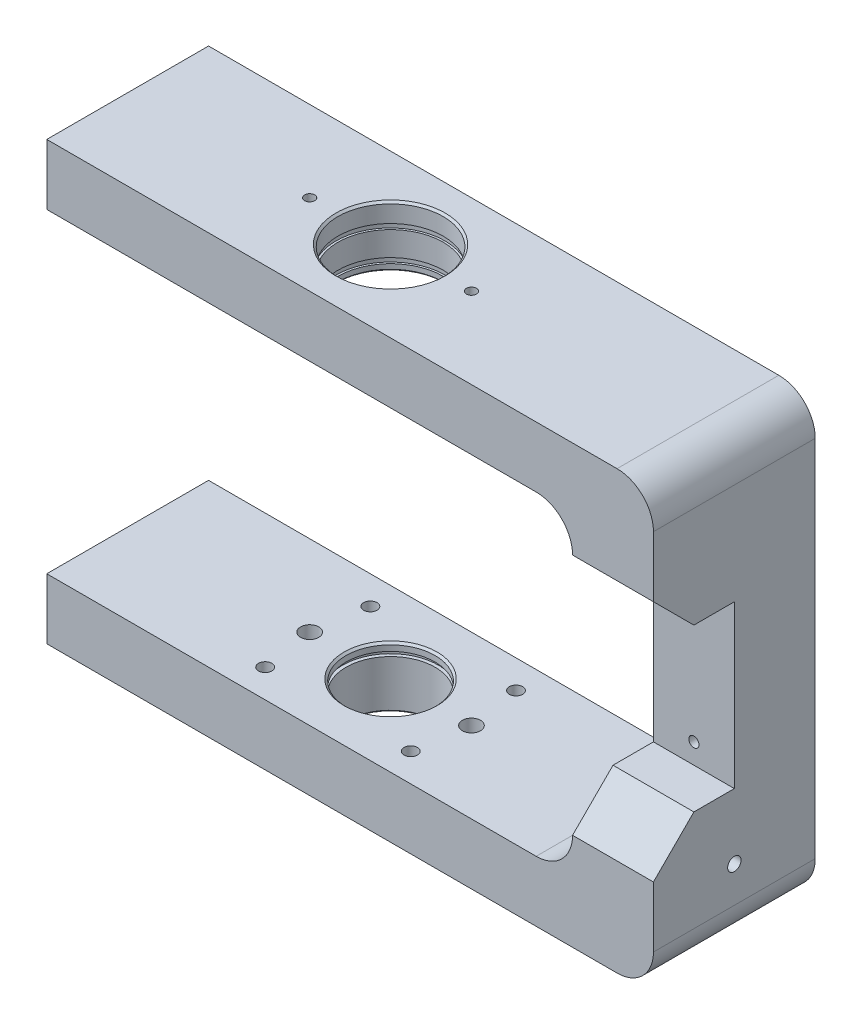
from build123d import *

# Parameters (mm, degrees)
BOSS_EXTRUDE1_DEPTH   = 40
SKETCH2_R             = 11
CUT_EXTRUDE1_DEPTH    = 190.1137224
SKETCH3_R             = 13
CUT_EXTRUDE2_DEPTH    = 40
SKETCH4_R             = 11.85
CUT_EXTRUDE3_DEPTH    = 1.1
SKETCH5_R             = 13.5
CUT_EXTRUDE4_DEPTH    = 1.3
LPATTERN1_COUNT       = 2
LPATTERN1_PITCH       = 7.3
M3_TAPPED_HOLE1_D     = 2.5
M3_TAPPED_HOLE1_DEPTH = 7.5
M3_TAPPED_HOLE1_TIP   = 0.751075774
CUT_EXTRUDE5_REACH    = 191.114
CHAMFER1_SIZE         = 0.5
M3_TAPPED_HOLE2_D     = 2.5
M3_TAPPED_HOLE2_DEPTH = 7.5
M3_TAPPED_HOLE2_TIP   = 0.751075774
M4_TAPPED_HOLE1_D     = 3.3
M4_TAPPED_HOLE1_DEPTH = 15.5
M4_TAPPED_HOLE1_TIP   = 0.991420021
SKETCH14_R            = 2.25
CUT_EXTRUDE6_DEPTH    = 24
M4_TAPPED_HOLE2_D     = 3.3
M4_TAPPED_HOLE2_DEPTH = 15


with BuildPart() as part:
    # Sketch1 → Boss-Extrude1 (new body)
    with BuildSketch(Plane.XY):
        with BuildLine():
            Line((0, 0), (141, 0))
            ThreePointArc((141, 0), (147.363961031, 2.636038969), (150, 9))
            Line((150, 9), (150, 99))
            ThreePointArc((150, 99), (147.363961031, 105.363961031), (141, 108))
            Line((141, 108), (0, 108))
            Line((0, 108), (0, 93))
            Line((0, 93), (121, 93))
            ThreePointArc((121, 93), (127.363961031, 90.363961031), (130, 84))
            Line((130, 84), (130, 24))
            ThreePointArc((130, 24), (127.363961031, 17.636038969), (121, 15))
            Line((121, 15), (0, 15))
            Line((0, 15), (0, 0))
        make_face()
    extrude(amount=BOSS_EXTRUDE1_DEPTH)

    # Sketch2 → Cut-Extrude1 (cut, through all)
    with BuildSketch(Plane(origin=(0, 108, 0), x_dir=(1, 0, 0), z_dir=(0, 1, 0))):
        with Locations(Location((65, -20, 0), (0, 0, 180))):
            Circle(SKETCH2_R)
    extrude(amount=-CUT_EXTRUDE1_DEPTH, mode=Mode.SUBTRACT)

    # Sketch3 → Cut-Extrude2 (cut)
    with BuildSketch(Plane(origin=(0, 108, 0), x_dir=(1, 0, 0), z_dir=(0, 1, 0))):
        with Locations(Location((65, -20, 0), (0, 0, 180))):
            Circle(SKETCH3_R)
    extrude(amount=-CUT_EXTRUDE2_DEPTH, mode=Mode.SUBTRACT)

    # Sketch4 → Cut-Extrude3 (cut)
    with BuildSketch(Plane(origin=(0, 12, 0), x_dir=(1, 0, 0), z_dir=(0, 1, 0))):
        with Locations(Location((65, -20, 0), (0, 0, 180))):
            Circle(SKETCH4_R)
    extrude(amount=CUT_EXTRUDE3_DEPTH, mode=Mode.SUBTRACT)

    # Sketch5 → Cut-Extrude4 (cut)
    with BuildSketch(Plane(origin=(0, 96, 0), x_dir=(-1, 0, 0), z_dir=(0, -1, 0))):
        with Locations(Location((-65, -20, 0), (0, 0, 90))):
            Circle(SKETCH5_R)
    cut_extrude4 = extrude(amount=CUT_EXTRUDE4_DEPTH, mode=Mode.SUBTRACT)

    # LPattern1: Cut-Extrude4 ×2
    with Locations(*[(0, i * LPATTERN1_PITCH, 0) for i in range(1, LPATTERN1_COUNT)]):
        add(cut_extrude4, mode=Mode.SUBTRACT)

    # M3 Tapped Hole1
    with Locations(Plane(origin=(45, 108, 20), x_dir=(1, 0, 0), z_dir=(0, 1, 0))):
        with Locations((0, 0), (40, 0)):
            Hole(M3_TAPPED_HOLE1_D / 2, depth=M3_TAPPED_HOLE1_DEPTH)
            with Locations((0, 0, -(M3_TAPPED_HOLE1_DEPTH + M3_TAPPED_HOLE1_TIP / 2))):  # 118° drill point
                Cone(0, M3_TAPPED_HOLE1_D / 2, M3_TAPPED_HOLE1_TIP, mode=Mode.SUBTRACT)

    # Sketch9 → Cut-Extrude5 (cut, up to next)
    with BuildSketch(Plane(origin=(150, 0, 0), x_dir=(0, 0, -1), z_dir=(1, 0, 0)), mode=Mode.PRIVATE) as cut_extrude5_sk1:
        Polygon((-40, 24), (-30, 34), (-20, 34), (-20, 74), (-30, 74), (-40, 84), align=None)
    cut_extrude5_tool1 = extrude(cut_extrude5_sk1.sketch, amount=-CUT_EXTRUDE5_REACH, mode=Mode.PRIVATE) & part.part
    add(cut_extrude5_tool1.solids().sort_by_distance((150, 54, 30.740741))[0], mode=Mode.SUBTRACT)

    # Chamfer1
    chamfer1_edges = [part.edges().sort_by_distance(p)[0] for p in [
        (76, 0, 20),
        (76, 15, 20),
        (78, 93, 20),
        (78, 108, 20),
    ]]
    chamfer(chamfer1_edges, length=CHAMFER1_SIZE)

    # M3 Tapped Hole2
    with Locations(Plane(origin=(140, 69, 20), x_dir=(1, 0, 0), z_dir=(0, 0, 1))):
        with Locations((0, 0), (0, -30)):
            Hole(M3_TAPPED_HOLE2_D / 2, depth=M3_TAPPED_HOLE2_DEPTH)
            with Locations((0, 0, -(M3_TAPPED_HOLE2_DEPTH + M3_TAPPED_HOLE2_TIP / 2))):  # 118° drill point
                Cone(0, M3_TAPPED_HOLE2_D / 2, M3_TAPPED_HOLE2_TIP, mode=Mode.SUBTRACT)

    # M4 Tapped Hole1
    with Locations(Plane(origin=(150, 17.860571099, 20), x_dir=(0, 0, 1), z_dir=(1, 0, 0))):
        with Locations((0, 0)):
            Hole(M4_TAPPED_HOLE1_D / 2, depth=M4_TAPPED_HOLE1_DEPTH)
            with Locations((0, 0, -(M4_TAPPED_HOLE1_DEPTH + M4_TAPPED_HOLE1_TIP / 2))):  # 118° drill point
                Cone(0, M4_TAPPED_HOLE1_D / 2, M4_TAPPED_HOLE1_TIP, mode=Mode.SUBTRACT)

    # Sketch14 → Cut-Extrude6 (cut)
    with BuildSketch(Plane.XZ):
        with Locations((85, 20)):
            Circle(SKETCH14_R)
        with Locations(Location((45, 20, 0), (0, 0, 270))):
            Circle(SKETCH14_R)
    extrude(amount=-CUT_EXTRUDE6_DEPTH, mode=Mode.SUBTRACT)

    # M4 Tapped Hole2
    with Locations(Plane(origin=(47, 0, 33), x_dir=(0, 0, -1), z_dir=(0, -1, 0))):
        with Locations((0, 0), (0, 36), (26, 36), (26, 0)):
            Hole(M4_TAPPED_HOLE2_D / 2, depth=M4_TAPPED_HOLE2_DEPTH)


solid = part.part
